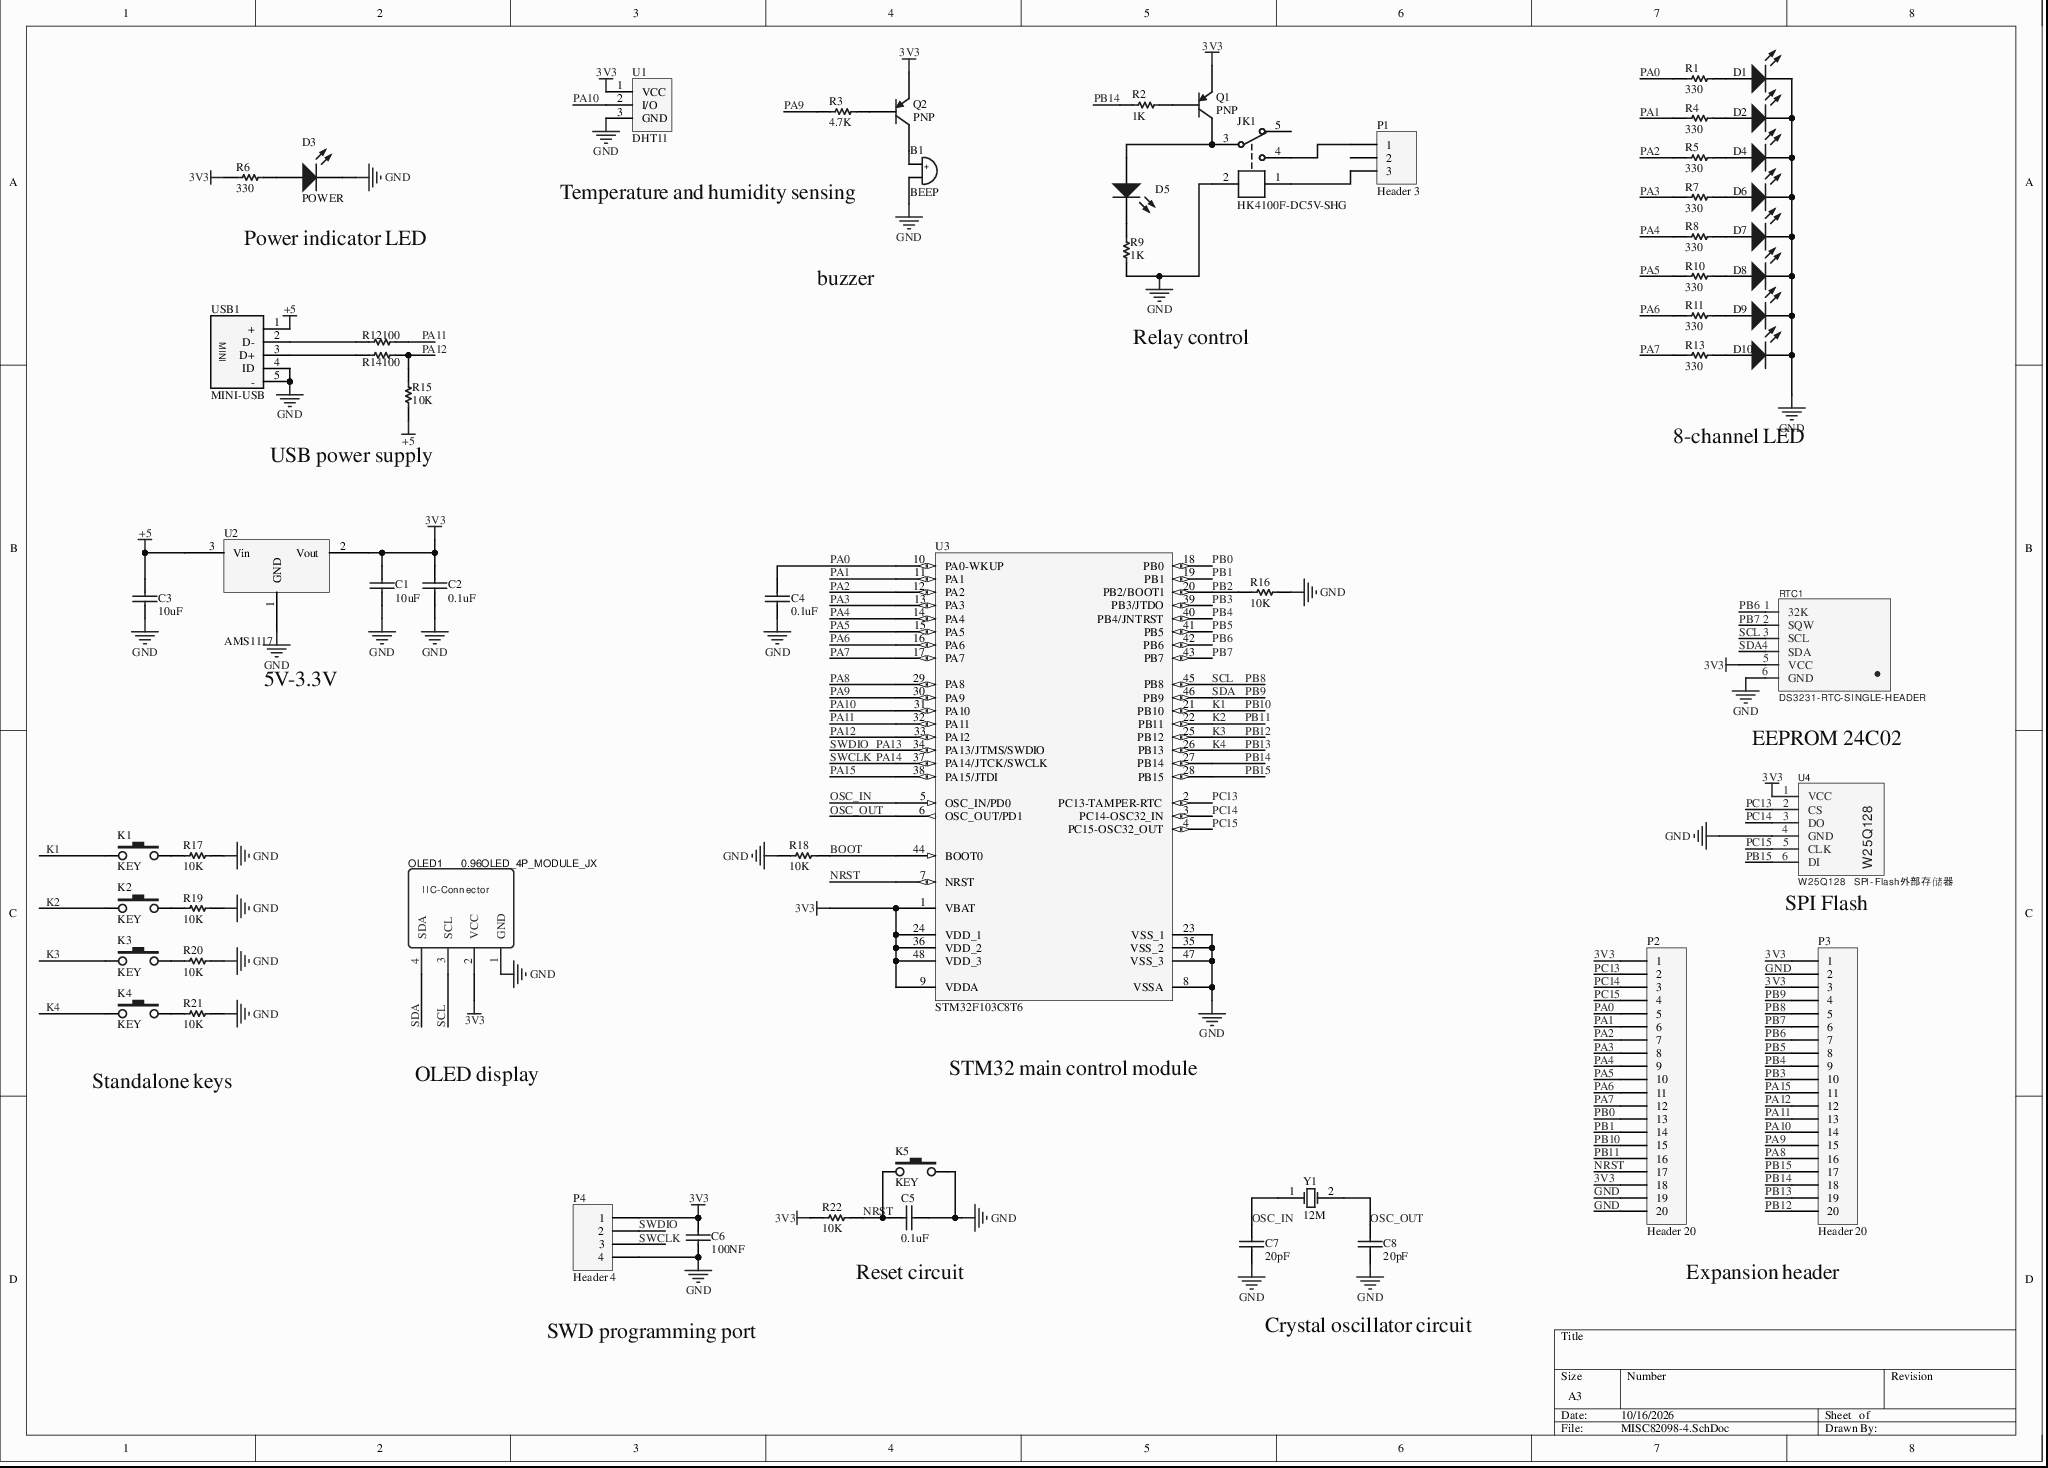
[diagram p0: MISC82098-4.SchDoc]
# Altium project MISC82098-7.PrjPcb
1 sheet, 61 parts. Net scope: global (net labels, ports and power ports of the same name join across sheets).
Board file: MISC82098.PcbDoc

## Sheet MISC82098-4.SchDoc
size A3

### Parts
B1  BEEP  [HDR1X2]
C1  10uF  [C0603]
C2  0.1uF  [C0603]
C3  10uF  [C0603]
C4  0.1uF  [C0603]
C5  0.1uF  [C0603]
C6  100NF  [C0603]
C7  20pF  [C0603]
C8  20pF  [C0603]
D1  POWER  [3.2X1.6X1.1]  (value not drawn)
D2  POWER  [3.2X1.6X1.1]  (value not drawn)
D3  POWER  [3.2X1.6X1.1]
D4  POWER  [3.2X1.6X1.1]  (value not drawn)
D5  POWER  [3.2X1.6X1.1]  (value not drawn)
D6  POWER  [3.2X1.6X1.1]  (value not drawn)
D7  POWER  [3.2X1.6X1.1]  (value not drawn)
D8  POWER  [3.2X1.6X1.1]  (value not drawn)
D9  POWER  [3.2X1.6X1.1]  (value not drawn)
D10  POWER  [3.2X1.6X1.1]  (value not drawn)
JK1  HK4100F-DC5V-SHG  [HK4100F]
K1  KEY  [DIP-3X6X4.3]
K2  KEY  [DIP-3X6X4.3]
K3  KEY  [DIP-3X6X4.3]
K4  KEY  [DIP-3X6X4.3]
K5  KEY  [DIP-3X6X4.3]
OLED1  0.96OLED_4P_MODULE_JX  [0.96OLED_4P]
P1  Header 3  [HDR1X3]
P2  Header 20  [HDR1X20]
P3  Header 20  [HDR1X20]
P4  Header 4  [HDR1X4]
Q1  PNP  [SOT-23B_N]
Q2  PNP  [SOT-23B_N]
R1  330  [6-0805_N]
R2  1K  [6-0805_N]
R3  4.7K  [6-0805_N]
R4  330  [6-0805_N]
R5  330  [6-0805_N]
R6  330  [6-0805_N]
R7  330  [6-0805_N]
R8  330  [6-0805_N]
R9  1K  [6-0805_N]
R10  330  [6-0805_N]
R11  330  [6-0805_N]
R12  100  [6-0805_N]
R13  330  [6-0805_N]
R14  100  [6-0805_N]
R15  10K  [6-0805_N]
R16  10K  [6-0805_N]
R17  10K  [6-0805_N]
R18  10K  [6-0805_N]
R19  10K  [6-0805_N]
R20  10K  [6-0805_N]
R21  10K  [6-0805_N]
R22  10K  [6-0805_N]
RTC1  DS3231-RTC-SINGLE-HEADER  [DS3231-RTC-24C32-EEPROM-SINGLE-HEADER]
U1  DHT11  [HDR1X3]
U2  AMS1117  [SOT223]
U3  STM32F103C8T6  [LQFP48 7X7]
U4  W25Q128  SPI-Flash外部存储器  [SPI FLASH]
USB1  MINI-USB  [USB-MINI-A]
Y1  12M  [XTAL_US]

### Nets
3V3: C1.2 C2.2 C6.2 OLED1.2(VCC) P2.1 P2.18 P3.1 P3.3 P4.1 Q1.3(E) Q2.3(E) R6.2 R22.2 RTC1.5(VCC) U1.1(VCC) U2.2(Vout) U3.1(VBAT) U3.9(VDDA) U3.24(VDD_1) U3.36(VDD_2) U3.48(VDD_3) U4.1(VCC)
+5: C3.2 R15.2 U2.3(Vin) USB1.1(+)
GND: B1.2 C1.1 C2.1 C3.1 C4.1 C5.1 C6.1 C7.1 C8.1 D1.2(K) D2.2(K) D3.2(K) D4.2(K) D6.2(K) D7.2(K) D8.2(K) D9.2(K) D10.2(K) JK1.2 K5.3 OLED1.1(GND) P2.19 P2.20 P3.2 P4.4 R9.2 R16.1 R17.1 R18.2 R19.1 R20.1 R21.1 RTC1.6(GND) U1.3(GND) U2.1(GND) U3.8(VSSA) U3.23(VSS_1) U3.35(VSS_2) U3.47(VSS_3) U4.4(GND) USB1.4(ID) USB1.5(-)
BOOT: R18.1 U3.44(BOOT0)
K1: K1.1 P2.15 U3.21(PB10)  [also labelled PB10]
K2: K2.1 P2.16 U3.22(PB11)  [also labelled PB11]
K3: K3.1 P3.20 U3.25(PB12)  [also labelled PB12]
K4: K4.1 P3.19 U3.26(PB13)  [also labelled PB13]
NRST: C5.2 K5.1 P2.17 R22.1 U3.7(NRST)
OSC_IN: C7.2 U3.5(OSC_IN/PD0) Y1.1(OSC1)
OSC_OUT: C8.2 U3.6(OSC_OUT/PD1) Y1.2(OSC2)
PA0: C4.2 P2.5 R1.2 U3.10(PA0-WKUP)
PA1: P2.6 R4.2 U3.11(PA1)
PA2: P2.7 R5.2 U3.12(PA2)
PA3: P2.8 R7.2 U3.13(PA3)
PA4: P2.9 R8.2 U3.14(PA4)
PA5: P2.10 R10.2 U3.15(PA5)
PA6: P2.11 R11.2 U3.16(PA6)
PA7: P2.12 R13.2 U3.17(PA7)
PA8: P3.16 U3.29(PA8)
PA9: P3.15 R3.2 U3.30(PA9)
PA10: P3.14 U1.2(I/O) U3.31(PA10)
PA11: P3.13 R12.1 U3.32(PA11)
PA12: P3.12 R14.1 R15.1 U3.33(PA12)
PA13: P4.2 U3.34(PA13/JTMS/SWDIO)  [also labelled SWDIO]
PA14: P4.3 U3.37(PA14/JTCK/SWCLK)  [also labelled SWCLK]
PA15: P3.11 U3.38(PA15/JTDI)
PB0: P2.13 U3.18(PB0)
PB1: P2.14 U3.19(PB1)
PB2: R16.2 U3.20(PB2/BOOT1)
PB3: P3.10 U3.39(PB3/JTDO)
PB4: P3.9 U3.40(PB4/JNTRST)
PB5: P3.8 U3.41(PB5)
PB6: P3.7 RTC1.1(32K) U3.42(PB6)
PB7: P3.6 RTC1.2(SQW) U3.43(PB7)
PB8: OLED1.3(SCL) P3.5 RTC1.3(SCL) U3.45(PB8)  [also labelled SCL]
PB9: OLED1.4(SDA) P3.4 RTC1.4(SDA) U3.46(PB9)  [also labelled SDA]
PB14: P3.18 R2.2 U3.27(PB14)
PB15: P3.17 U3.28(PB15) U4.6(DI)
PC13: P2.2 U3.2(PC13-TAMPER-RTC) U4.2(CS)
PC14: P2.3 U3.3(PC14-OSC32_IN) U4.3(DO)
PC15: P2.4 U3.4(PC15-OSC32_OUT) U4.5(CLK)
NetB1_1: B1.1 Q2.1(C)
NetD1_1: D1.1(A) R1.1
NetD2_1: D2.1(A) R4.1
NetD3_1: D3.1(A) R6.1
NetD4_1: D4.1(A) R5.1
NetD5_1: D5.1(A) JK1.3 Q1.1(C)
NetD5_2: D5.2(K) R9.1
NetD6_1: D6.1(A) R7.1
NetD7_1: D7.1(A) R8.1
NetD8_1: D8.1(A) R10.1
NetD9_1: D9.1(A) R11.1
NetD10_1: D10.1(A) R13.1
NetJK1_1: JK1.1 P1.3
NetJK1_4: JK1.4 P1.1
NetK1_3: K1.3 R17.2
NetK2_3: K2.3 R19.2
NetK3_3: K3.3 R20.2
NetK4_3: K4.3 R21.2
NetQ1_2: Q1.2(B) R2.1
NetQ2_2: Q2.2(B) R3.1
NetR12_2: R12.2 USB1.2(D-)
NetR14_2: R14.2 USB1.3(D+)

Not connected (* = marked no-connect by the designer): JK1 5; P1 2

### Notes on the sheet
- (near B1) Temperature and humidity sensing
- Power indicator LED
- buzzer
- Relay control
- (near R15) USB power supply
- 8-channel LED
- 5V-3.3V
- EEPROM 24C02
- SPI Flash
- Standalone keys
- OLED display
- STM32 main control module
- Reset circuit
- Expansion header
- SWD programming port
- Crystal oscillator circuit

### Library data of the parts
B1 = BEEP: buzzer
C1-C8 = CAP: non-polarized capacitor
D1-D10 = LED2: Typical RED, GREEN, YELLOW, AMBER GaAs LED; Published: 8-Jun-2000; LatestRevisionDate: 17-Jul-2002; LatestRevisionNote: Re-released for DXP Platform.; PackageVersion: Feb-2002; PackageReference: 3.2X1.6X1.1; PackageDescription: SM LED; 2 Flat Leads; Publisher: Altium Limited
JK1 = HK4100F: changeover switch set
OLED1 = 0.96OLED_4P_MODULE_JX: Manufacturer: null; Contributor: LCSC; Supplier: LCSC; Supplier Part: C9900004566; Manufacturer Part: 0.96OLED_4P_MODULE_JX; JLCPCB Part Class: Extended Part; spicePre: O; spiceSymbolName: 0.96OLED_4P_MODULE_JX
P1 U1 = Header 3: Header, 3-Pin; LatestRevisionDate: 17-Jul-2002; LatestRevisionNote: Re-released for DXP Platform.; Publisher: Altium Limited
P2 P3 = Header 20: Header, 20-Pin; LatestRevisionDate: 17-Jul-2002; LatestRevisionNote: Re-released for DXP Platform.; Publisher: Altium Limited
P4 = Header 4: Header, 4-Pin; LatestRevisionDate: 17-Jul-2002; LatestRevisionNote: Re-released for DXP Platform.; Publisher: Altium Limited
Q1 Q2 = PNP: PNP Bipolar Transistor; Published: 8-Jun-2000; LatestRevisionDate: 29-May-2009; LatestRevisionNote: IPC-7351 Footprint Added.; PackageVersion: Aug-1999; PackageReference: SOT-23B; PackageDescription: 3-Pin SOT-23 Package 0.95 mm Pitch, 2.4 mm Lead Span; Publisher: Altium Limited
R1-R22 = RES
U2 = AMS1117: three-terminal voltage regulator
Y1 = XTAL: Crystal Oscillator; Published: 8-Jun-2000; LatestRevisionDate: 17-Jul-2002; LatestRevisionNote: Re-released for DXP Platform.; Publisher: Altium Limited